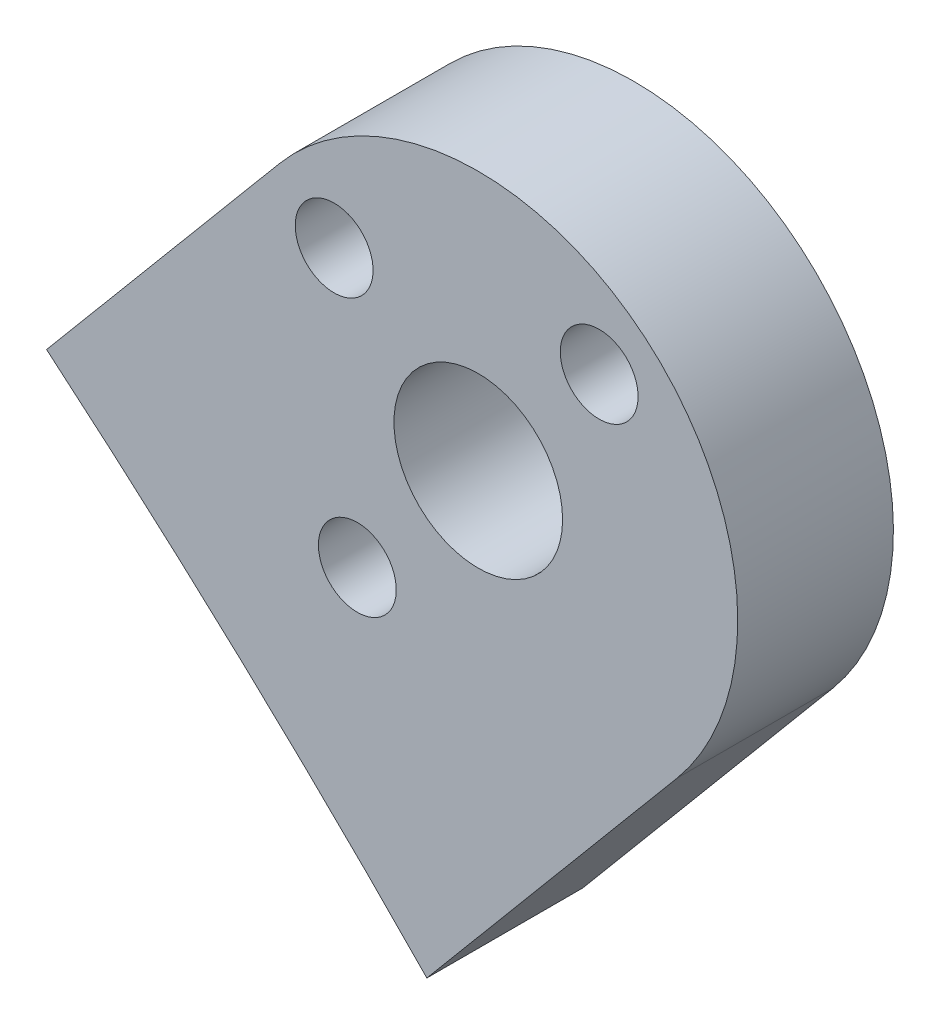
SolidWorks part; units mm, degrees
material "钢板12/Q235A"
ref_plane "Front Plane" through (0, 0, 0) normal (0, 0, 1) x (1, 0, 0)
ref_plane "Top Plane" through (0, 0, 0) normal (0, 1, 0) x (1, 0, 0)
ref_plane "Right Plane" through (0, 0, 0) normal (1, 0, 0) x (0, 0, -1)
sketch "Sketch1" plane through (0, 0, 0) normal (0, 0, 1) x (1, 0, 0)
  line L0 (0, 0) -> (0, 387.5) construction
  line L1 (0, 0) -> (249.0802, 296.8422) construction
  line L2 (249.0802, 296.8422) -> (267.0332, 318.2378)
  line L3 (278.3914, 269.545) -> (297.675, 292.5263)
  line L4 (282.3541, 305.3821) -> (264.0887, 283.5726) construction
  circle A0 centre (0, 0) radius 387.5 construction
  arc A1 (267.0332, 318.2378) -> (297.675, 292.5263) centre (282.3541, 305.3821) cw
  arc A2 (249.0802, 296.8422) -> (278.3914, 269.545) centre (0, 0) cw
  circle A3 centre (282.3541, 305.3821) radius 6.5
  dimension "D1" = 775
  dimension "D3" = 20
  dimension "D5" = 13
  dimension "D2" = 40
  dimension "D4" = 30
  dimension "D6" = 40
extrude "Boss-Extrude1" add sketch "Sketch1" along normal mid plane 12
sketch "Sketch2" plane through (0, 0, -6) normal (0, 0, -1) x (-1, 0, 0)
  line L0 (-282.3541, 305.3821) -> (-295.2099, 320.7029) construction
  arc A0 (-267.0332, 318.2378) -> (-297.675, 292.5263) centre (-282.3541, 305.3821) ccw construction
  circle A7 centre (-282.3541, 305.3821) radius 14.5 construction
  circle A8 centre (-291.6745, 316.4897) radius 3
  circle A9 centre (-271.2465, 314.7025) radius 3
  circle A10 centre (-273.0337, 294.2744) radius 3
  circle A11 centre (-293.4618, 296.0616) radius 3 construction
  point P17 (-282.3541, 305.3821)
  dimension "D1" = 29
  dimension "D2" = 6
  dimension "D3" = 4
extrude "Cut-Extrude1" cut sketch "Sketch2" against normal up to surface (12 mm away) up to face at (276.3471, 298.2128, 6)
cosmetic thread "Cosmetic Thread1" parameters "D2"=6.8
cosmetic thread "Cosmetic Thread2" parameters "D2"=6.8
cosmetic thread "Cosmetic Thread3" parameters "D2"=6.8
